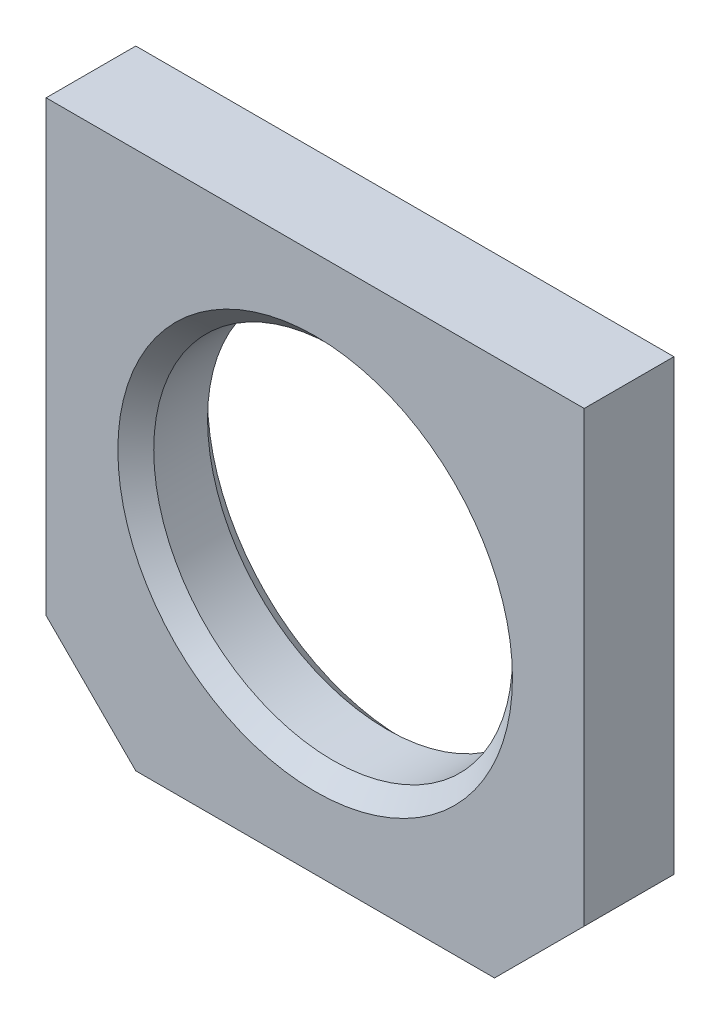
from build123d import *

# Parameters (mm, degrees)
SKETCH_1_W      = 60
SKETCH_1_H      = 60
SKETCH_1_R      = 20
EXTRUDE_1_DEPTH = 10
CHAMFER_1_SIZE  = 10
CHAMFER_3_SIZE  = 2


with BuildPart() as part:
    # 草图1 → 凸台-拉伸1 (new body)
    with BuildSketch(Plane.XY):
        Rectangle(SKETCH_1_W, SKETCH_1_H)
        Circle(SKETCH_1_R, mode=Mode.SUBTRACT)
    extrude(amount=EXTRUDE_1_DEPTH)

    # 倒角1
    chamfer_1_edges = [part.edges().sort_by_distance(p)[0] for p in [
        (30, -30, 5),
        (-30, -30, 5),
    ]]
    chamfer(chamfer_1_edges, length=CHAMFER_1_SIZE)

    # 倒角3
    chamfer_3_edges = [part.edges().sort_by_distance(p)[0] for p in [
        (-20, 0, 0),
        (-20, 0, 10),
    ]]
    chamfer(chamfer_3_edges, length=CHAMFER_3_SIZE)


solid = part.part
